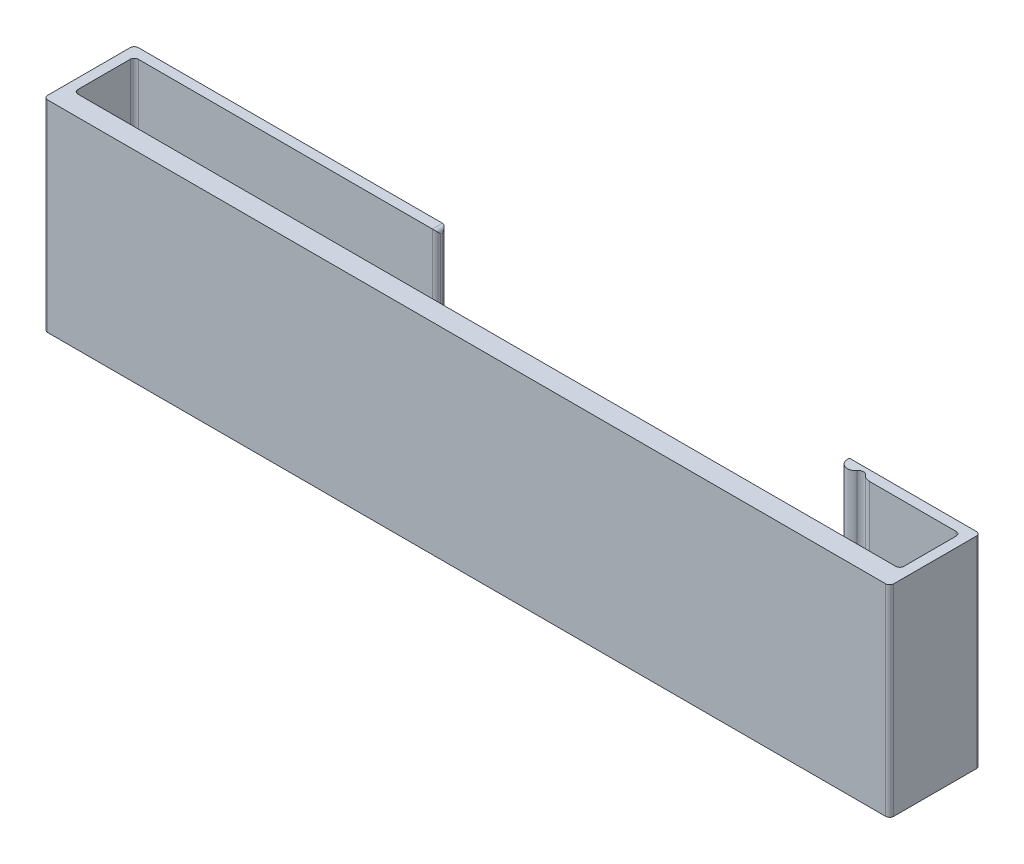
SolidWorks part; units mm, degrees
material "1.4000 (X6Cr13)"
ref_plane "Front Plane" through (0, 0, 0) normal (0, 0, 1) x (1, 0, 0)
ref_plane "Top Plane" through (0, 0, 0) normal (0, 1, 0) x (1, 0, 0)
ref_plane "Right Plane" through (0, 0, 0) normal (1, 0, 0) x (0, 0, -1)
sketch "Sketch1" plane through (0, 0, 0) normal (0, 0, 1) x (1, 0, 0)
  line L0 (-127.0312, 120.619) -> (-127.0312, 110.619) construction
  line L1 (-142.5312, 120.619) -> (-100.5312, 120.619) construction
  line L2 (-142.5312, 120.619) -> (-142.5312, 110.619) construction
  line L3 (-142.5312, 110.619) -> (-100.5312, 110.619) construction
  line L4 (-100.5312, 120.619) -> (-100.5312, 110.619) construction
  line L5 (-142.5312, 120.619) -> (-100.5312, 110.619) construction
  line L6 (-142.5312, 110.619) -> (-100.5312, 120.619) construction
  line L8 (-142.5312, 120.619) -> (-127.0312, 120.619)
  line L9 (-142.5312, 120.619) -> (-142.5312, 110.619)
  line L10 (-142.5312, 110.619) -> (-127.0312, 110.619)
  line L11 (-127.0312, 120.619) -> (-127.0312, 110.619)
  point P0 (-121.5312, 115.619)
  dimension "D1" = 10
  dimension "D2" = 42
  dimension "D3" = 26.5
extrude "Boss-Extrude1" add sketch "Sketch1" along normal blind 0.5
sketch "Sketch2" plane through (0, 0, 0.5) normal (0, 0, 1) x (1, 0, 0)
  line L1 (-142.5312, 120.619) -> (-142.0312, 120.619)
  line L2 (-142.5312, 120.619) -> (-142.5312, 110.619)
  line L3 (-142.5312, 110.619) -> (-142.0312, 110.619)
  line L4 (-142.0312, 120.619) -> (-142.0312, 110.619)
  line L5 (-142.5312, 110.619) -> (-127.0312, 110.619) construction
  dimension "D1" = 0.5
extrude "Boss-Extrude2" add sketch "Sketch2" along normal blind 3
sketch "Sketch3" plane through (0, 0, 3.5) normal (0, 0, 1) x (1, 0, 0)
  line L0 (-121.5312, 120.619) -> (-121.5312, 80.6369) construction
  line L1 (-142.5312, 120.619) -> (-100.5312, 120.619)
  line L2 (-142.5312, 120.619) -> (-142.5312, 110.619)
  line L3 (-142.5312, 110.619) -> (-100.5312, 110.619)
  line L4 (-100.5312, 120.619) -> (-100.5312, 110.619)
  dimension "D1" = 21
  dimension "D2" = 10
extrude "Boss-Extrude3" add sketch "Sketch3" along normal blind 1
sketch "Sketch4" plane through (0, 0, 4.5) normal (0, 0, 1) x (1, 0, 0)
  line L1 (-100.5312, 120.619) -> (-101.0312, 120.619)
  line L2 (-100.5312, 120.619) -> (-100.5312, 110.619)
  line L3 (-100.5312, 110.619) -> (-101.0312, 110.619)
  line L4 (-101.0312, 120.619) -> (-101.0312, 110.619)
  line L5 (-142.5312, 110.619) -> (-100.5312, 110.619) construction
  dimension "D1" = 0.5
extrude "Boss-Extrude4" add sketch "Sketch4" against normal blind 4.5
sketch "Sketch6" plane through (0, 110.619, 0) normal (0, -1, 0) x (-1, 0, 0)
  line L0 (100.5312, 0) -> (107.0312, 0)
  line L1 (106.2083, 0) -> (136.854, 0) construction
  line L2 (107.0312, 0) -> (107.0312, -0.1)
  line L3 (105.5312, -0.5) -> (100.5312, -0.5)
  line L4 (100.5312, -4.5) -> (100.5312, 0) construction
  line L5 (100.5312, -0.5) -> (100.5312, 0)
  line L6 (105.0312, 0) -> (138.0312, 0) construction
  arc A0 (106.3077, -0.3353) -> (105.9141, -0.3216) centre (106.1055, -0.4823) ccw
  arc A1 (106.3077, -0.3353) -> (107.0312, -0.1) centre (106.6312, -0.1) ccw
  arc A2 (105.5312, -0.5) -> (105.9141, -0.3216) centre (105.5312, 0) ccw
  dimension "D1" = 0.5
  dimension "D2" = 0.8
  dimension "D3" = 0.5
  dimension "D4" = 0.5
  dimension "D5" = 6.5
  dimension "D6" = 5
extrude "Boss-Extrude5" add sketch "Sketch6" against normal up to surface (10 mm away) up to face at (-122.6312, 120.619, 1.7)
fillet "Fillet1" radius 0.2 12 edges at (-127.0312, 110.619, 0.25) (-127.0312, 115.619, 0.5) (-127.0312, 120.619, 0.25) (-127.0312, 115.619, 0) (-101.0312, 115.619, 0.5) (-101.0312, 115.619, 3.5) (-100.5312, 115.619, 0) (-100.5312, 115.619, 4.5) (-142.0312, 115.619, 0.5) (-142.0312, 115.619, 3.5) (-142.5312, 115.619, 0) (-142.5312, 115.619, 4.5)
